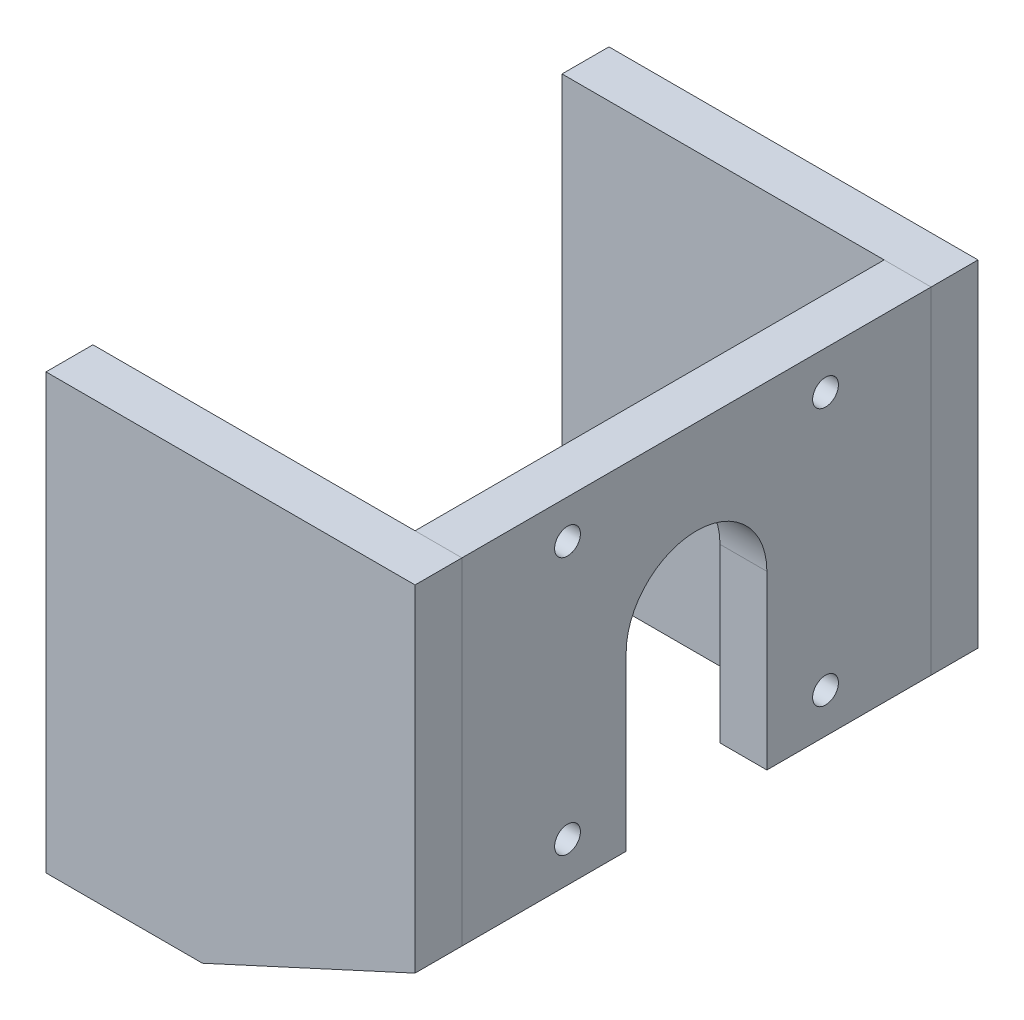
SolidWorks part; units mm, degrees
other "Markup1"
sketch "草图7" plane through (125, -137.5, -260) normal (0.9291, -0.2477, -0.2748) x (-0.292, -0.0351, -0.9558)
material "普通碳钢"
ref_plane "Front Plane" through (0, 0, 0) normal (0, 0, 1) x (1, 0, 0)
ref_plane "Top Plane" through (0, 0, 0) normal (0, 1, 0) x (1, 0, 0)
ref_plane "Right Plane" through (0, 0, 0) normal (1, 0, 0) x (0, 0, -1)
other "Configuration Table"
sketch "Sketch1" plane through (0, 0, 0) normal (0, 0, 1) x (1, 0, 0)
  line L0 (-118, 138.75) -> (-118, -138.75)
  line L2 (118, -76.25) -> (118, 138.75)
  line L5 (-127.9813, 0) -> (393.3982, 0) construction
  line L7 (-18, -138.75) -> (-118, -138.75)
  line L9 (-18, -138.75) -> (118, -76.25)
  line L11 (118, 138.75) -> (-118, 138.75)
  dimension "D1" = 277.5
  dimension "D2" = 236
  dimension "D3" = 215
  dimension "D4" = 100
extrude "Boss-Extrude1" add sketch "Sketch1" along normal blind 30
ref_plane "Plane1" through (0, 0, -150) normal (0, 0, -1) x (-1, 0, 0)
mirror "Mirror2" about plane through (0, 0, -150) normal (0, 0, -1) of bodies 106 107
sketch "Sketch5" plane through (0, 0, 0) normal (1, 0, 0) x (0, 0, -1)
  line L5 (150, -163.1461) -> (150, 145.4216) construction
  line L7 (150, -129.8) -> (150, 129.8) construction
  line L9 (195, 33.75) -> (195, -76.25)
  line L12 (0, 138.75) -> (150, 138.75)
  line L13 (0, 138.75) -> (0, -76.25)
  line L14 (0, -76.25) -> (105, -76.25)
  line L15 (300, 138.75) -> (300, -76.25)
  line L17 (195, -76.25) -> (300, -76.25)
  line L20 (150, 138.75) -> (300, 138.75)
  line L21 (105, 33.75) -> (105, -76.25)
  arc A2 (105, 33.75) -> (195, 33.75) centre (150, 33.75) ccw construction
  circle A11 centre (67.5, 114.25) radius 8.25
  circle A12 centre (232.5, 114.25) radius 8.25
  circle A13 centre (232.5, -50.75) radius 8.25
  circle A14 centre (67.5, -50.75) radius 8.25
  arc A15 (195, 33.75) -> (105, 33.75) centre (150, 33.75) ccw
  dimension "D1" = 45
  dimension "D8" = 165
  dimension "D3" = 16.5
  dimension "D5" = 165
  dimension "D2" = 110
  dimension "D4" = 67.5
  dimension "D7" = 25.5
extrude "Boss-Extrude2" add sketch "Sketch5" against normal blind 30 from surface at 118 separate body starting at face at (118, 31.25, 15)
